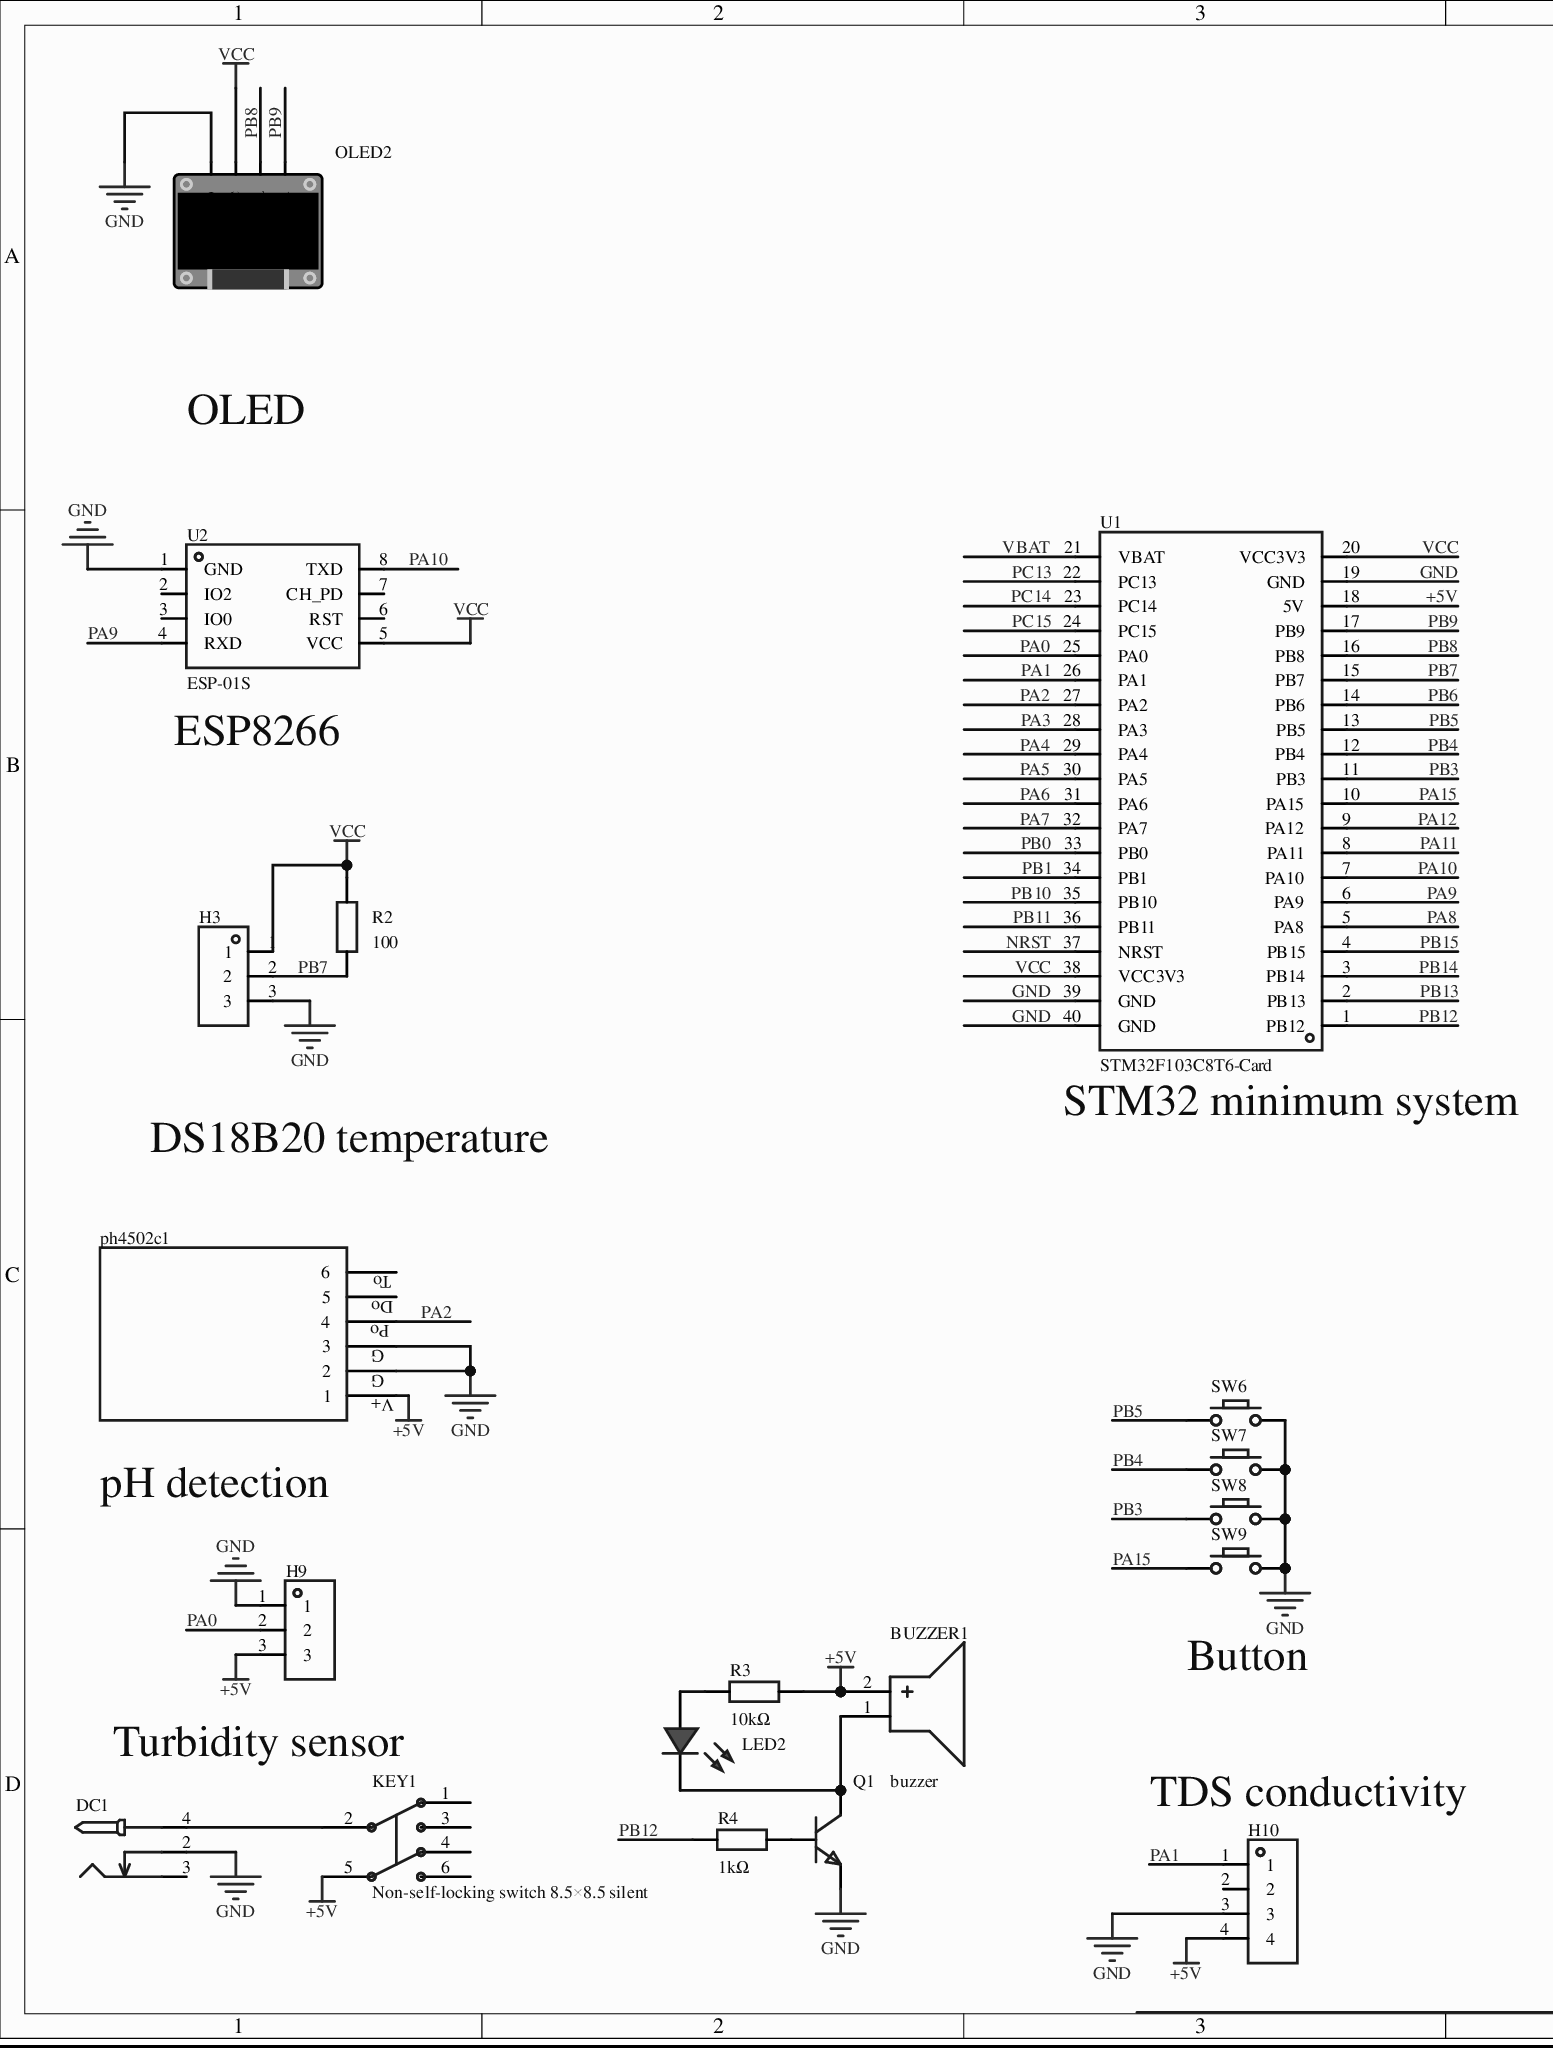
[diagram p0: MISC49912-3.schdoc]
# Altium project MISC49912-2.PrjPcb
1 sheet, 19 parts. Net scope: global (net labels, ports and power ports of the same name join across sheets).
Board file: MISC49912.pcbdoc

## Sheet MISC49912-3.schdoc
size 297 x 209 mm; Version: V1.0; @Project Name: MISC49912; @Page Count: 1; @Update Date: 2026-05-11; @Create Date: 2026-05-11; @Schematic Name: MISC49912; @Page No: 1; @Create Time: 23:22:16; @Update Time: 17:32:40; @Board Name: MISC49912

### Parts
BUZZER1  buzzer  [BUZ-TH_BD12.0-P6.00-D0.9-RD]
DC1  (no value)  [DC-2.0]
H3  (no value)  [HDR-TH_3P-P2.54-V-F]
H9  (no value)  [HDR-TH_3P-P2.54-V-F]
H10  (no value)  [HDR-TH_4P-P2.54-V-F]
KEY1  Non-self-locking switch 8.5×8.5 silent  [SW-TH_6P-L8.5-W8.5-P2.54]
LED2  (no value)  [LED_TH-3mm]
OLED2  (no value)  [0.96OLED_4P]
ph4502c1  (no value)  [PH4502C]
Q1  (no value)  [S8050_TO_92]
R2  100  [Res_1/8W]
R3  10kΩ  [Res_1/8W]
R4  1kΩ  [Res_1/8W]
SW6  (no value)  [Key_TH_3.5x6x4.3]
SW7  (no value)  [Key_TH_3.5x6x4.3]
SW8  (no value)  [Key_TH_3.5x6x4.3]
SW9  (no value)  [Key_TH_3.5x6x4.3]
U1  STM32F103C8T6-Card  [CONN-TH_L53.3-W22.9_STM32F103C8T6-CARD]
U2  ESP-01S  [WIFIM-TH_ESP-01S]

### Nets
+5V: BUZZER1.2(+) H9.3 H10.4 KEY1.5 ph4502c1.1 R3.2 U1.18(5V)
GND: DC1.2 H3.3 H9.1 H10.3 OLED2.1(GND) ph4502c1.2 ph4502c1.3 Q1.1(E) SW6.B SW7.B SW8.B SW9.B U1.19(GND) U1.39(GND) U1.40(GND) U2.1(GND)
VCC: H3.1 OLED2.2(VCC) R2.2 U1.20(VCC3V3) U1.38(VCC3V3) U2.5(VCC)
NRST: U1.37(NRST)
PA0: H9.2 U1.25(PA0)
PA1: H10.1 U1.26(PA1)
PA2: ph4502c1.4 U1.27(PA2)
PA3: U1.28(PA3)
PA4: U1.29(PA4)
PA5: U1.30(PA5)
PA6: U1.31(PA6)
PA7: U1.32(PA7)
PA8: U1.5(PA8)
PA9: U1.6(PA9) U2.4(RXD)
PA10: U1.7(PA10) U2.8(TXD)
PA11: U1.8(PA11)
PA12: U1.9(PA12)
PA15: SW9.A U1.10(PA15)
PB0: U1.33(PB0)
PB1: U1.34(PB1)
PB3: SW8.A U1.11(PB3)
PB4: SW7.A U1.12(PB4)
PB5: SW6.A U1.13(PB5)
PB6: U1.14(PB6)
PB7: H3.2 R2.1 U1.15(PB7)
PB8: OLED2.3(SCL) U1.16(PB8)
PB9: OLED2.4(SDA) U1.17(PB9)
PB10: U1.35(PB10)
PB11: U1.36(PB11)
PB12: R4.1 U1.1(PB12)
PB13: U1.2(PB13)
PB14: U1.3(PB14)
PB15: U1.4(PB15)
PC13: U1.22(PC13)
PC14: U1.23(PC14)
PC15: U1.24(PC15)
VBAT: U1.21(VBAT)
NetBUZZER1_1: BUZZER1.1(-) LED2.2(A) Q1.3(C)
NetDC1_4: DC1.4 KEY1.2
NetLED2_1: LED2.1(C) R3.1
NetQ1_2: Q1.2(B) R4.2

Not connected (* = marked no-connect by the designer): DC1 3; H10 2*; KEY1 1 3 4 6; ph4502c1 5* 6*; U2 2(IO2)* 3(IO0)* 6(RST)* 7(CH_PD)*

### Notes on the sheet
- OLED
- (near U2) ESP8266
- DS18B20 temperature
- (near U1) STM32 minimum system
- pH detection
- (near SW9) Button
- Turbidity sensor
- (near H10) TDS conductivity

### Library data of the parts
BUZZER1 = buzzer: AddInBom: yes; ModelId: af17e4151ed84fc2a628230bf23763630819f05c4eef4c71ace90d822a990e87; ModelTransform: 472.44,472.176,0,270,0,0,0,0,-196.85; Symbol: BUZZER; Device: buzzer; LCSC Part Name: buzzer; SupplierPart: C9900014030; ManufacturerPart: buzzer; Supplier Footprint: buzzer; JLCPCB Part Class: Extended Part; Supplier: LCSC; ConvertToPcb: yes; FootprintName: BUZ-TH_BD12.0-P6.00-D0.9-RD; ModelName: BUZ-TH_BD12.0-P6.00-D0.9-RD
DC1 = DC-005_2.0: Symbol: DC power jack; ConvertToPcb: yes; ModelId: f5f20b8a2308479b936ba3c2698865bb0819f05c4eef4c71ace90d822a990e87; ModelName: DC-IN-TH_DC-5520-1; ModelTransform: 372.05,551.18,582.68,90,0,0,137.8,0,-149.61; Device: DC-005_2.0; AddInBom: yes; Supplier Footprint: 插件; FootprintName: DC-2.0
H3 H9 = HDR-F_2.54_1x3P: Symbol: PM254V-11-03-H85; ConvertToPcb: yes; ModelId: f3b3cc5aae9641bf9e56fc160cef875b; ModelName: HDR2.54-F-LI-1X3P; ModelTransform: 299.9994,100,0,0,0,0,0,0,-118.11; Device: HDR-F_2.54_1x3P; FootprintName: HDR-TH_3P-P2.54-V-F; AddInBom: yes; SupplierPart: C541850; Supplier Footprint: 插件
H10 = HDR-F_2.54_1x4P: Symbol: 2.54-1*4P female; ConvertToPcb: yes; ModelId: d187812051054f85879fcaa51a310d8e0819f05c4eef4c71ace90d822a990e87; ModelTransform: 419.6842,98.464,0,0,0,0,0,0,-118.11; Device: HDR-F_2.54_1x4P; AddInBom: yes; SupplierPart: C2718488; Supplier Footprint: 插件; FootprintName: HDR-TH_4P-P2.54-V-F; ModelName: HDR-TH_4P-P2.54-V-F
KEY1 = 无自锁开关 8.5×8.5 无声: 6脚，8.5×8.5; Symbol: No self-locking switch 8.5×8.5 silent; AddInBom: yes; ModelId: 4c72b3966b92446eb355e1bd0fb4f8800819f05c4eef4c71ace90d822a990e87; ModelTransform: 342.519,334.645,0,180,0,0,0,0,-137.795; Device: Non-self-locking switch 8.5×8.5 silent; LCSC Part Name: 无自锁开关 8.5×8.5  无声; SupplierPart: C26228; ManufacturerPart: 无自锁开关 8.5×8.5 无声; Supplier Footprint: 插件; JLCPCB Part Class: Extended Part; Supplier: LCSC; ConvertToPcb: yes; FootprintName: SW-TH_6P-L8.5-W8.5-P2.54; ModelName: SW-TH_6P-L8.5-W8.5-P2.54
LED2 = LED_TH-R_3mm: 3D Model: a497c992633541038a38947cdc58012f0819f05c4eef4c71ace90d822a990e87; 3D Model Transform: 141.274,153.327,0,0,0,0,-5.984,0,-137.795; ConvertToPcb: yes; ModelName: LED-TH-3mm_R; Symbol: LED_TH-R; Device: LED_TH-R_3mm; Supplier Footprint: 插件; AddInBom: yes; FootprintName: LED_TH-3mm
OLED2 = 0.96OLED模块_4P: Symbol: 0.96OLED module_4P; ConvertToPcb: yes; ModelId: 79c000fdb68d45a296c2e9bedf4f9055; ModelTransform: 1393.69792,1318.895,0,0,0,0,0,-560.079,-137.795; Device: 0.96OLED module_4P; AddInBom: yes; FootprintName: 0.96OLED_4P; Supplier Footprint: 插件; ModelName: 0.96OLED_4P
ph4502c1 = PH4502C: Symbol: ESP32 dev board_1; AddInBom: yes; Device: PH4502C; ConvertToPcb: yes; FootprintName: PH4502C
Q1 = S8050_TO_NPN: ConvertToPcb: yes; ModelId: aafe8e06f2154e7c93506efd0d6632dd; ModelName: TO-92-3_L4.9-W3.7-P1.27-L; ModelTransform: 180.78,141.44,417.3,0,0,0,0,0,-200; Symbol: S8050_TO_NPN; Device: S8050_TO_NPN; AddInBom: yes; Supplier Footprint: TO-92; FootprintName: S8050_TO_92
R2-R4 = Res_AXIAL-1/8W: Symbol: Resistor; 3D Model: b2b5ae7ae4c642178fe0039925c86a3f0819f05c4eef4c71ace90d822a990e87; 3D Model Transform: 282.86,66.88,253.09,0,0,0,0,0,-191; ConvertToPcb: yes; ModelName: RES-TH_BD1.8-L3.2-P7.20-D0.4; Device: Res_AXIAL-1/8W; Supplier Footprint: 轴向引线; AddInBom: yes; FootprintName: Res_1/8W
  R2: Value: 100
  R3: Value: 10kΩ
  R4: Value: 1kΩ
SW6-SW9 = Key_TH_3.5x6x4.3: ConvertToPcb: yes; ModelId: c3523f9014d949d7ba5445190a3178990819f05c4eef4c71ace90d822a990e87; ModelName: SW-TH_L6.0-W3.5-H5.0-P6.5; ModelTransform: 308.49,137.8,335.08,0,0,0,0,0,-129.92; Symbol: Key_TH_3.5x6x4.3; Device: Key_TH_3.5x6x4.3; AddInBom: yes; Supplier Footprint: 插件; FootprintName: Key_TH_3.5x6x4.3
U1 = STM32F103C8T6-Card: AddInBom: yes; Device: STM32F103C8T6-Card; Symbol: STM32F103C8T6-CARD; FootprintName: CONN-TH_L53.3-W22.9_STM32F103C8T6-CARD; LCSC Part Name: STM32F103C8T6-Card; SupplierPart: C9900077949; ManufacturerPart: STM32F103C8T6-Card; Supplier Footprint: 插件; Supplier: LCSC; ConvertToPcb: yes
U2 = ESP-01S_C111009: AddInBom: yes; ModelId: eb7175da78ae48b3b1568cfe3027405f0819f05c4eef4c71ace90d822a990e87; ModelTransform: 582.676,976.37608,0,0,0,0,0,388.346,-118.11; Symbol: ESP-01S; Device: ESP-01S_C111009; LCSC Part Name: ESP-01S; SupplierPart: C111009; ManufacturerPart: ESP-01S; Supplier Footprint: -; JLCPCB Part Class: Extended Part; Supplier: LCSC; ConvertToPcb: yes; FootprintName: WIFIM-TH_ESP-01S; ModelName: WIFIM-TH_ESP-01S